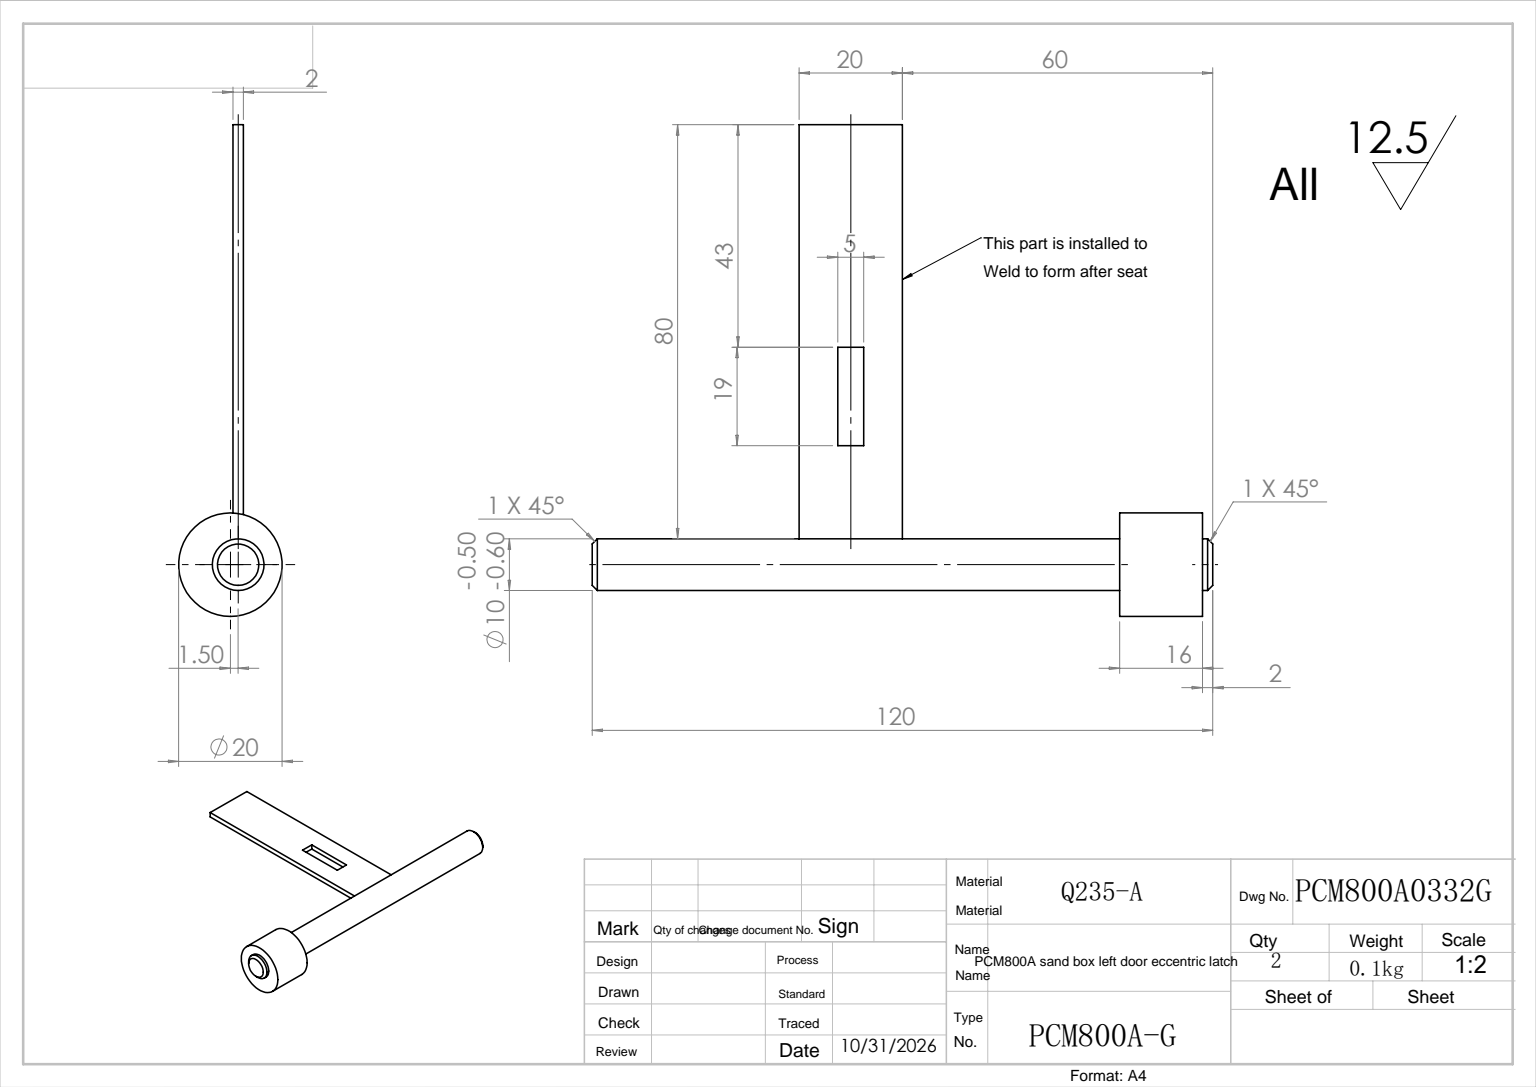
from build123d import *

# Parameters (mm, degrees)
SKETCH_1_R      = 5
EXTRUDE_1_DEPTH = 120
EXTRUDE_START   = -2
SKETCH_2_R      = 10
EXTRUDE_2_DEPTH = 16
SKETCH_3_W      = 80
SKETCH_3_H      = 20
SKETCH_3_W_2    = 19
SKETCH_3_H_2    = 5
EXTRUDE_3_DEPTH = 1
CHAMFER_1_SIZE  = 1


with BuildPart() as part:
    # 草图1 → 凸台-拉伸1 (new body)
    with BuildSketch(Plane.XY):
        Circle(SKETCH_1_R)
    extrude(amount=EXTRUDE_1_DEPTH)

    # 草图2 → 凸台-拉伸2 (add)
    with BuildSketch(Plane.XY.offset(120).offset(EXTRUDE_START)):
        with Locations((0, -1.5)):
            Circle(SKETCH_2_R)
    extrude(amount=-EXTRUDE_2_DEPTH)

    # 倒角1
    chamfer_1_edges = [part.edges().sort_by_distance(p)[0] for p in [
        (-5, 0, 0),
        (-5, 0, 120),
    ]]
    chamfer(chamfer_1_edges, length=CHAMFER_1_SIZE)


with BuildPart() as body_2:
    # 草图3 → 凸台-拉伸3 (new, symmetric)
    with BuildSketch(Plane(origin=(0, 0, 0), x_dir=(1, 0, 0), z_dir=(0, 1, 0))):
        with Locations((-45, -50)):
            Rectangle(SKETCH_3_W, SKETCH_3_H)
        with Locations((-32.5, -50)):
            Rectangle(SKETCH_3_W_2, SKETCH_3_H_2, mode=Mode.SUBTRACT)
    extrude(amount=EXTRUDE_3_DEPTH, both=True)


solid = Compound([part.part, body_2.part])
